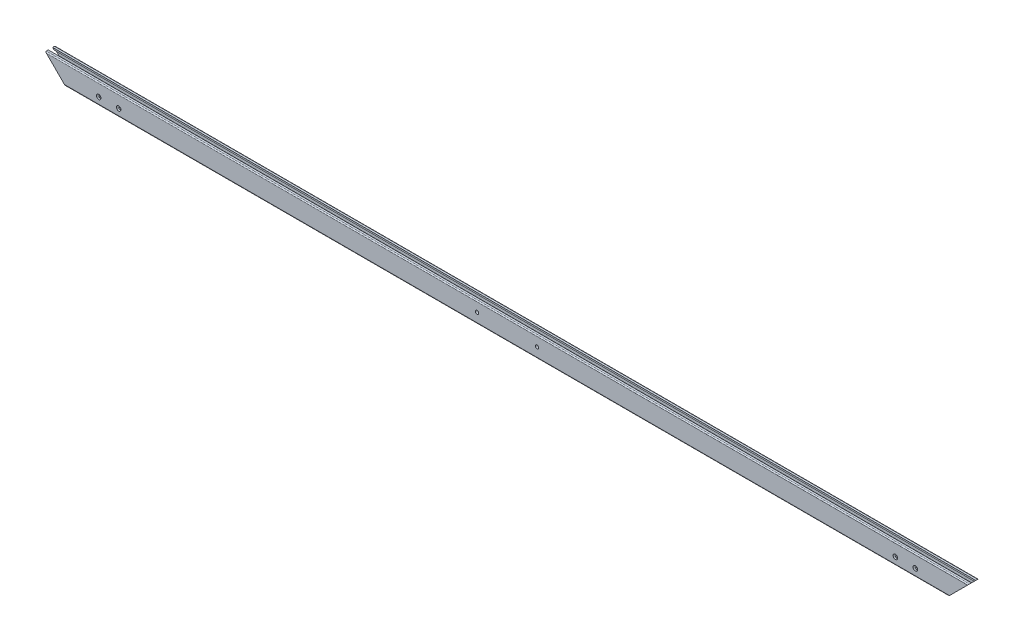
from build123d import *

# Parameters (mm, degrees)
SKETCH11_R             = 2.5
MEMBER_1_DEPTH         = 1386
CUT_EXTRUDE_1_DEPTH    = 694.324599304
HOLE_WIZARD_M8_1_D     = 6.8
HOLE_WIZARD_M6_1_D     = 5
HOLE_WIZARD_M6_1_DEPTH = 17
HOLE_WIZARD_M6_1_TIP   = 1.502151548


with BuildPart() as part:
    # Sketch11 → Member 1 (new body)
    with BuildSketch(Plane(origin=(-693, 0, 0), x_dir=(0, 0, -1), z_dir=(1, 0, 0))):
        with BuildLine():
            Line((-6, -15), (-3.25, -15))
            Line((-3.25, -15), (-3.25, -12.7))
            Line((-3.25, -12.7), (-5, -12.7))
            Line((-5, -12.7), (-5, -7))
            ThreePointArc((-5, -7), (0, -4.31662479), (5, -7))
            Line((5, -7), (5, -12.7))
            Line((5, -12.7), (3.25, -12.7))
            Line((3.25, -12.7), (3.25, -15))
            Line((3.25, -15), (6, -15))
            ThreePointArc((6, -15), (7.060660172, -14.560660172), (7.5, -13.5))
            Line((7.5, -13.5), (7.5, 13.5))
            ThreePointArc((7.5, 13.5), (7.060660172, 14.560660172), (6, 15))
            Line((6, 15), (3.25, 15))
            Line((3.25, 15), (3.25, 12.7))
            Line((3.25, 12.7), (5, 12.7))
            Line((5, 12.7), (5, 7))
            ThreePointArc((5, 7), (0, 4.31662479), (-5, 7))
            Line((-5, 7), (-5, 12.7))
            Line((-5, 12.7), (-3.25, 12.7))
            Line((-3.25, 12.7), (-3.25, 15))
            Line((-3.25, 15), (-6, 15))
            ThreePointArc((-6, 15), (-7.060660172, 14.560660172), (-7.5, 13.5))
            Line((-7.5, 13.5), (-7.5, -13.5))
            ThreePointArc((-7.5, -13.5), (-7.060660172, -14.560660172), (-6, -15))
        make_face()
        Circle(SKETCH11_R, mode=Mode.SUBTRACT)
    extrude(amount=MEMBER_1_DEPTH)

    # 草图4 → 切除-拉伸1 (cut, through all)
    with BuildSketch(Plane.XY.offset(7.5)):
        Polygon((-693, 15), (-663, -15), (-693, -15), align=None)
        Polygon((693, -15), (693, 15), (663, -15), align=None)
    extrude(amount=-CUT_EXTRUDE_1_DEPTH, mode=Mode.SUBTRACT)

    # M8 螺纹孔1 (through all)
    with Locations(Plane.XY.offset(7.5)):
        with Locations((-613, -4), (-583, -4), (583, -4), (613, -4)):
            Hole(HOLE_WIZARD_M8_1_D / 2)

    # M6 螺纹孔1
    with Locations(Plane.XY.offset(7.5)):
        with Locations((-45, 0), (45, 0)):
            Hole(HOLE_WIZARD_M6_1_D / 2, depth=HOLE_WIZARD_M6_1_DEPTH)
            with Locations((0, 0, -(HOLE_WIZARD_M6_1_DEPTH + HOLE_WIZARD_M6_1_TIP / 2))):  # 118° drill point
                Cone(0, HOLE_WIZARD_M6_1_D / 2, HOLE_WIZARD_M6_1_TIP, mode=Mode.SUBTRACT)


solid = part.part
